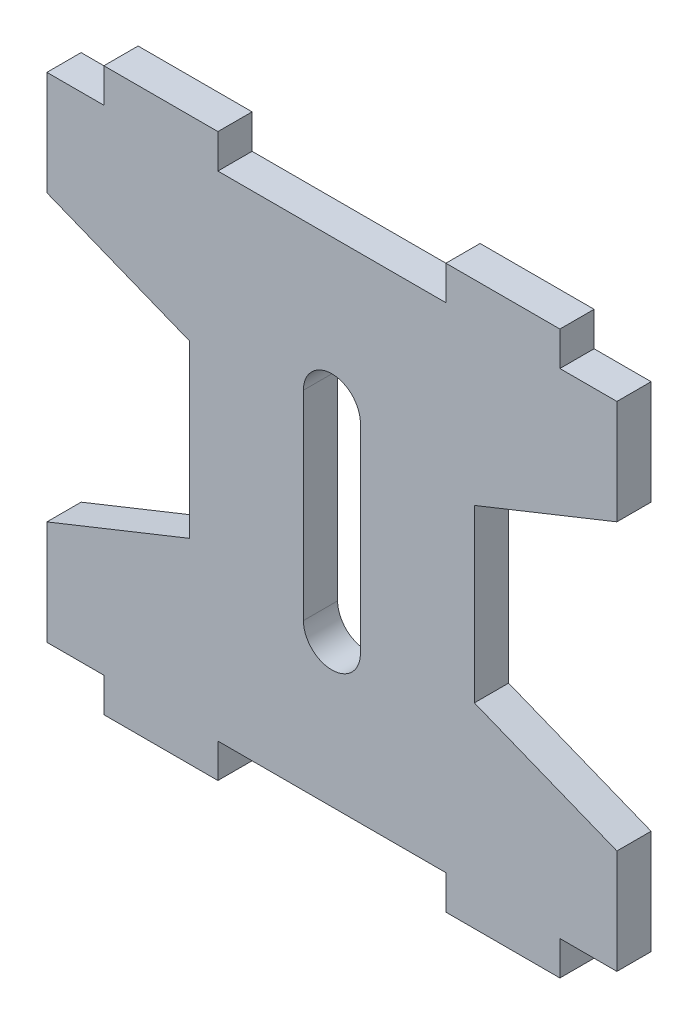
SolidWorks part; units mm, degrees
ref_plane "前视基准面" through (0, 0, 0) normal (0, 0, 1) x (1, 0, 0)
ref_plane "上视基准面" through (0, 0, 0) normal (0, 1, 0) x (1, 0, 0)
ref_plane "右视基准面" through (0, 0, 0) normal (1, 0, 0) x (0, 0, -1)
other "Configuration Table"
sketch "草图1" plane through (0, 0, 0) normal (0, 0, 1) x (1, 0, 0)
  line L0 (-73.5714, 0) -> (94.3024, 0) construction
  line L1 (0, 58.4629) -> (0, -59.4575) construction
  line L2 (-25.6092, -21.7689) -> (-20.6092, -21.7689)
  line L3 (-25.6092, -21.7689) -> (-25.6092, -12.6189)
  line L4 (-25.6092, 21.5311) -> (-20.6092, 21.5311)
  line L5 (24.3908, -21.7689) -> (24.3908, -12.6189)
  line L6 (-25.6092, -21.7689) -> (24.3908, 21.5311) construction
  line L7 (-25.6092, 21.5311) -> (24.3908, -21.7689) construction
  line L8 (-25.6092, 12.3811) -> (-13.1092, 7.3811)
  line L9 (-13.1092, 7.3811) -> (-13.1092, -7.6189)
  line L10 (-13.1092, -7.6189) -> (-25.6092, -12.6189)
  line L11 (-20.6092, 21.5311) -> (-20.6092, 24.5311)
  line L12 (-20.6092, 24.5311) -> (-10.6092, 24.5311)
  line L13 (-10.6092, 24.5311) -> (-10.6092, 21.5311)
  line L14 (-0.6092, 8.6311) -> (-0.6092, -8.8689) construction
  line L15 (1.8908, 8.6311) -> (1.8908, -8.8689)
  line L16 (-3.1092, 8.6311) -> (-3.1092, -8.8689)
  line L17 (11.8908, -7.6189) -> (24.3908, -12.6189)
  line L18 (11.8908, 7.3811) -> (11.8908, -7.6189)
  line L19 (24.3908, 12.3811) -> (11.8908, 7.3811)
  line L20 (9.3908, 24.5311) -> (9.3908, 21.5311)
  line L21 (19.3908, 24.5311) -> (9.3908, 24.5311)
  line L22 (19.3908, 21.5311) -> (19.3908, 24.5311)
  line L23 (19.3908, -21.7689) -> (19.3908, -24.7689)
  line L24 (19.3908, -24.7689) -> (9.3908, -24.7689)
  line L25 (9.3908, -24.7689) -> (9.3908, -21.7689)
  line L26 (-10.6092, -24.7689) -> (-10.6092, -21.7689)
  line L27 (-20.6092, -24.7689) -> (-10.6092, -24.7689)
  line L28 (-20.6092, -21.7689) -> (-20.6092, -24.7689)
  line L29 (-25.6092, 12.3811) -> (-25.6092, 21.5311)
  line L30 (24.3908, 12.3811) -> (24.3908, 21.5311)
  line L31 (-10.6092, 21.5311) -> (9.3908, 21.5311)
  line L32 (19.3908, 21.5311) -> (24.3908, 21.5311)
  line L33 (19.3908, -21.7689) -> (24.3908, -21.7689)
  line L34 (-10.6092, -21.7689) -> (9.3908, -21.7689)
  arc A0 (1.8908, 8.6311) -> (-3.1092, 8.6311) centre (-0.6092, 8.6311) ccw
  arc A1 (-3.1092, -8.8689) -> (1.8908, -8.8689) centre (-0.6092, -8.8689) ccw
  point P5 (-0.6092, -0.1189)
  point P20 (-0.6092, -0.1189)
  dimension "D7" = 2.5
  dimension "D1" = 50
  dimension "D2" = 43.3
  dimension "D3" = 12.5
  dimension "D4" = 3
  dimension "D5" = 10
  dimension "D6" = 5
  dimension "D8" = 17.5
extrude "凸台-拉伸1" add sketch "草图1" along normal blind 3 contours L15 A1 L16 A0 | L2 L28 L27 L26 L34 L25 L24 L23 L33 L5 L17 L18 L19 L30 L32 L22 L21 L20 L31 L13 L12 L11 L4 L29 L8 L9 L10 L3
